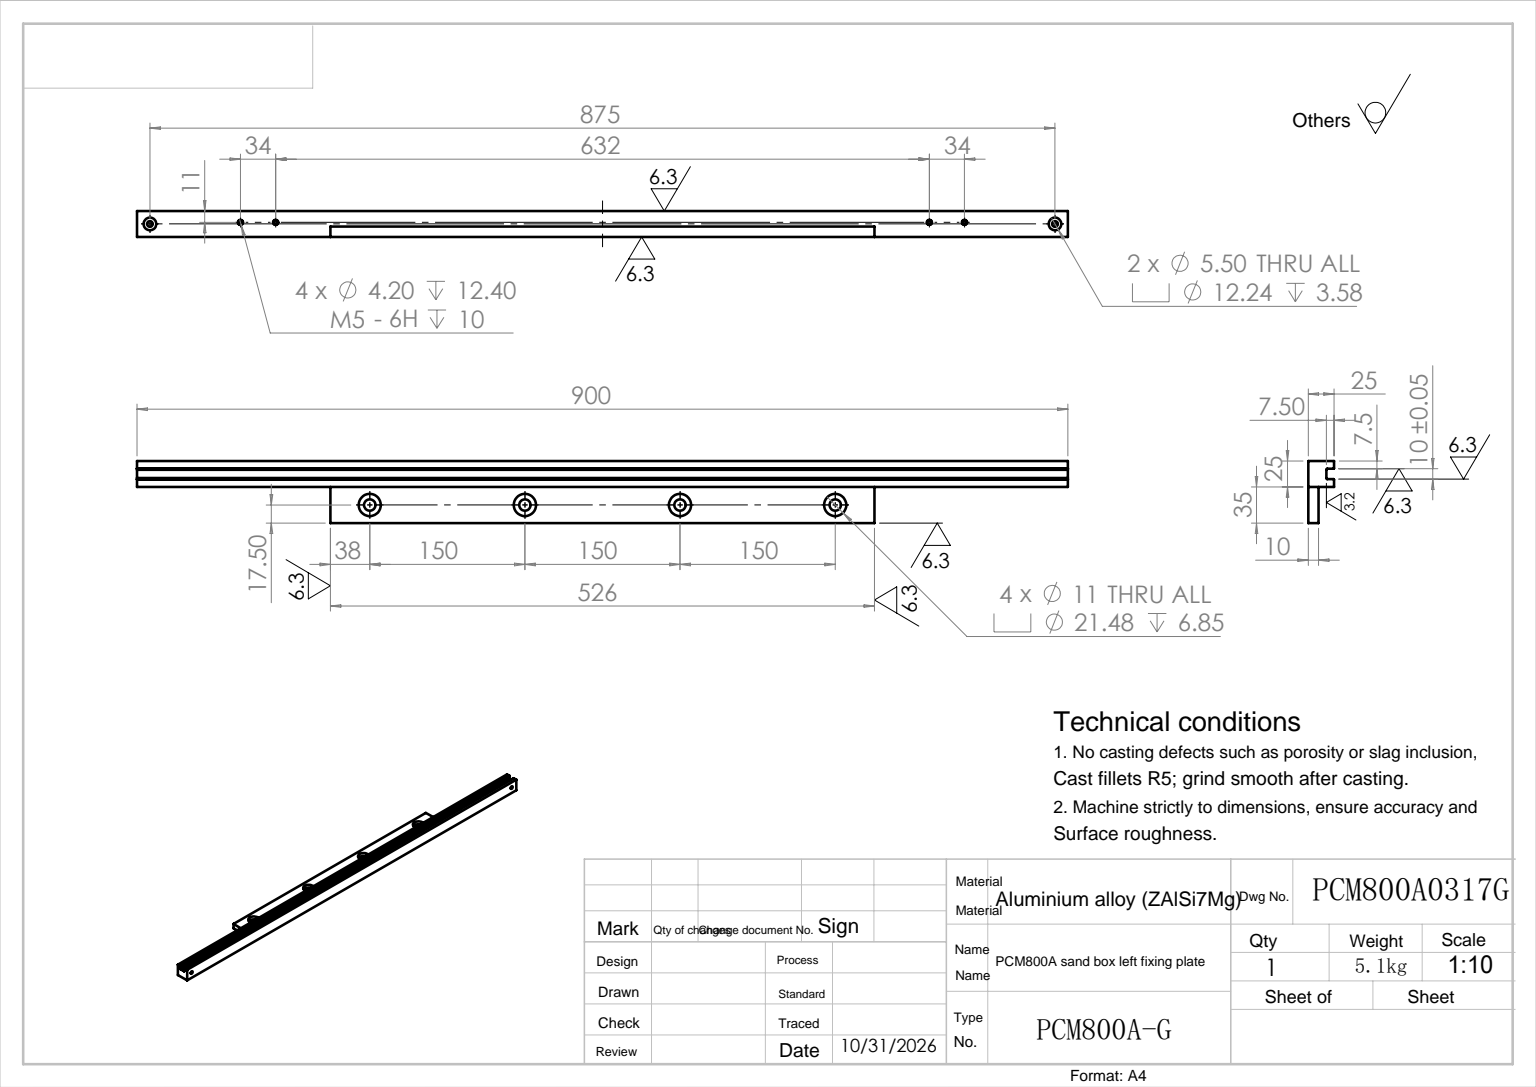
from build123d import *

# Parameters (mm, degrees)
SKETCH_1_W                    = 900
SKETCH_1_H                    = 25
EXTRUDE_1_DEPTH               = 25
SKETCH_2_W                    = 526
SKETCH_2_H                    = 10
EXTRUDE_2_DEPTH               = 35
CUT_EXTRUDE_1_DEPTH           = 902.027191599
CHAMFER_1_SIZE                = 0.5
HOLE_WIZARD_M10_1_D           = 11
HOLE_WIZARD_M10_1_CBORE_D     = 21.48
HOLE_WIZARD_M10_1_CBORE_DEPTH = 6.85
HOLE_WIZARD_M5_1_D            = 5.5
HOLE_WIZARD_M5_1_CBORE_D      = 12.24
HOLE_WIZARD_M5_1_CBORE_DEPTH  = 3.58
HOLE_WIZARD_M5_1_2_AT_2_COUNT = 2
HOLE_WIZARD_M5_1_2_AT_2_PITCH = 34
PATTERN_LINEAR_1_COUNT        = 2
PATTERN_LINEAR_1_PITCH        = 666


with BuildPart() as part:
    # 草图1 → 拉伸1 (new body)
    with BuildSketch(Plane(origin=(0, 0, 0), x_dir=(0, 0, -1), z_dir=(1, 0, 0))):
        with Locations((450, 12.5)):
            Rectangle(SKETCH_1_W, SKETCH_1_H)
    extrude(amount=EXTRUDE_1_DEPTH)

    # 草图2 → 拉伸2 (add)
    with BuildSketch(Plane.ZY):
        with Locations((-450, 5)):
            Rectangle(SKETCH_2_W, SKETCH_2_H)
    extrude(amount=EXTRUDE_2_DEPTH)

    # 草图3 → 切除-拉伸1 (cut, through all)
    with BuildSketch(Plane.XY):
        with BuildLine():
            Line((7.5, 25), (17.5, 25))
            Line((17.5, 25), (17.5, 18.5))
            ThreePointArc((17.5, 18.5), (17.207106781, 17.792893219), (16.5, 17.5))
            Line((16.5, 17.5), (8.5, 17.5))
            ThreePointArc((8.5, 17.5), (7.792893219, 17.792893219), (7.5, 18.5))
            Line((7.5, 18.5), (7.5, 25))
        make_face()
    extrude(amount=-CUT_EXTRUDE_1_DEPTH, mode=Mode.SUBTRACT)

    # 倒角1
    chamfer_1_edges = [part.edges().sort_by_distance(p)[0] for p in [
        (17.5, 25, -450),
        (7.5, 25, -450),
    ]]
    chamfer(chamfer_1_edges, length=CHAMFER_1_SIZE)

    # M10 六角头螺栓的柱形沉头孔1 (through all)
    with Locations(Plane(origin=(-17.5, 10, -675), x_dir=(0, 0, 1), z_dir=(0, 1, 0))):
        with Locations((0, 0), (150.000000001, 0), (300.000000001, 0), (450, 0)):
            CounterBoreHole(HOLE_WIZARD_M10_1_D / 2, HOLE_WIZARD_M10_1_CBORE_D / 2, HOLE_WIZARD_M10_1_CBORE_DEPTH)

    # Hole Wizard M5 _1 (through all)
    with Locations(Plane(origin=(0, 12.5, -887.5), x_dir=(0, 0, -1), z_dir=(-1, 0, 0))):
        with Locations((0, 0), (-875, 0)):
            CounterBoreHole(HOLE_WIZARD_M5_1_D / 2, HOLE_WIZARD_M5_1_CBORE_D / 2, HOLE_WIZARD_M5_1_CBORE_DEPTH)

    # 草图8 → Hole Wizard M5 _1 2 (revolve, cut)
    with BuildSketch(Plane(origin=(0, 14, -800), x_dir=(0, 0, 1), z_dir=(0, 1, 0))):
        Polygon((0, 0), (0, 13.6618073), (2.1, 12.4), (2.1, 10), (2.5, 10), (2.5, 0), align=None)
    hole_wizard_m5_1_2 = revolve(axis=Axis((-6.35, 14, -800), (1, 0, 0)), mode=Mode.SUBTRACT)

    # Hole Wizard M5 _1 2 at 2: Hole Wizard M5 _1 2 ×2
    with Locations(*[(0, 0, i * HOLE_WIZARD_M5_1_2_AT_2_PITCH) for i in range(1, HOLE_WIZARD_M5_1_2_AT_2_COUNT)]):
        add(hole_wizard_m5_1_2, mode=Mode.SUBTRACT)

    # 阵列(线性)1: Hole Wizard M5 _1 2 ×2
    with Locations(*[(0, 0, i * PATTERN_LINEAR_1_PITCH) for i in range(1, PATTERN_LINEAR_1_COUNT)]):
        add(hole_wizard_m5_1_2, mode=Mode.SUBTRACT)

    # 阵列(线性)1 copy 1 sketch → 阵列(线性)1 copy 1 (revolve, cut)
    with BuildSketch(Plane(origin=(0, 14, -100), x_dir=(0, 0, 1), z_dir=(0, 1, 0))):
        Polygon((0, 0), (0, 13.6618073), (2.1, 12.4), (2.1, 10), (2.5, 10), (2.5, 0), align=None)
    revolve(axis=Axis((-6.35, 14, -100), (1, 0, 0)), mode=Mode.SUBTRACT)


solid = part.part
